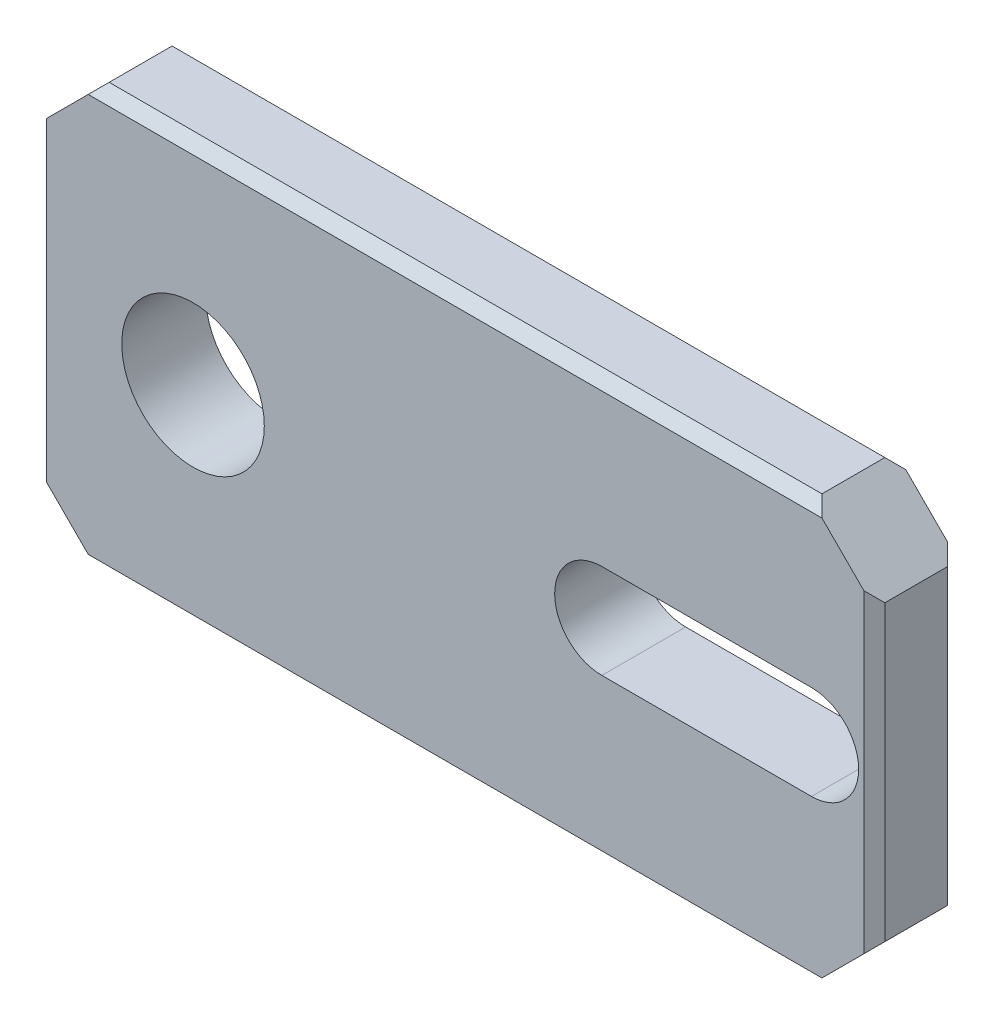
SolidWorks part; units mm, degrees
material "A6061"
ref_plane "Front Plane" through (0, 0, 0) normal (0, 0, 1) x (1, 0, 0)
ref_plane "Top Plane" through (0, 0, 0) normal (0, 1, 0) x (1, 0, 0)
ref_plane "Right Plane" through (0, 0, 0) normal (1, 0, 0) x (0, 0, -1)
sketch "Sketch1" plane through (0, 0, 0) normal (0, 0, 1) x (1, 0, 0)
  line L1 (-20, -10) -> (20, -10)
  line L2 (-20, -10) -> (-20, 10)
  line L3 (-20, 10) -> (20, 10)
  line L4 (20, -10) -> (20, 10)
  line L5 (-20, -10) -> (20, 10) construction
  line L6 (-20, 10) -> (20, -10) construction
  point P0 (0, 0)
  dimension "D1" = 40
  dimension "D2" = 20
extrude "Boss-Extrude1" add sketch "Sketch1" along normal blind 4
hole_wizard "M8 Tapped Hole1" positions "Sketch3" profile "Sketch2" tap size "M8" standard "GB" end condition through all
sketch "Sketch3" plane through (0, 0, 4) normal (0, 0, 1) x (1, 0, 0)
  line L0 (-20, 10) -> (-20, -10) construction
  line L1 (22.7728, 0) -> (-24.1132, 0) construction
  point P0 (-12.5, 0)
  dimension "D1" = 7.5
cosmetic thread "Cosmetic Thread1" parameters "D2"=8
sketch "Sketch2" plane through (-12.5, 0, 4) normal (1, 0, 0) x (0, -1, 0)
  line L0 (0, 0) -> (0, 4)
  line L1 (0, 4) -> (3.4, 4)
  line L2 (3.4, 4) -> (3.4, 0)
  line L5 (3.4, 0) -> (0, 0)
  line L11 (0, -6.35) -> (0, 107.95) construction
  dimension "通孔螺纹孔钻头直径" = 6.8
  dimension "通孔螺纹孔钻头深度" = 4
sketch "Sketch4" plane through (0, 0, 4) normal (0, 0, 1) x (1, 0, 0)
  line L0 (7, 0) -> (17, 0) construction
  line L1 (7, 2.25) -> (17, 2.25)
  line L2 (7, -2.25) -> (17, -2.25)
  line L3 (20, -10) -> (20, 10) construction
  arc A0 (7, 2.25) -> (7, -2.25) centre (7, 0) ccw
  arc A1 (17, -2.25) -> (17, 2.25) centre (17, 0) ccw
  point P3 (12, 0)
  dimension "D1" = 4.5
  dimension "D2" = 10
  dimension "D3" = 3
extrude "Cut-Extrude1" cut sketch "Sketch4" against normal blind 4
chamfer "Chamfer1" distance 3 angle 45 4 edges at (20, -10, 2) (-20, -10, 2) (-20, 10, 2) (20, 10, 2)
chamfer "Chamfer2" distance 0.5 angle 45 8 edges at (20, 0, 0) (20, 0, 4) (-20, 0, 4) (-20, 0, 0) (0, -10, 0) (0, -10, 4) (0, 10, 0) (0, 10, 4)
